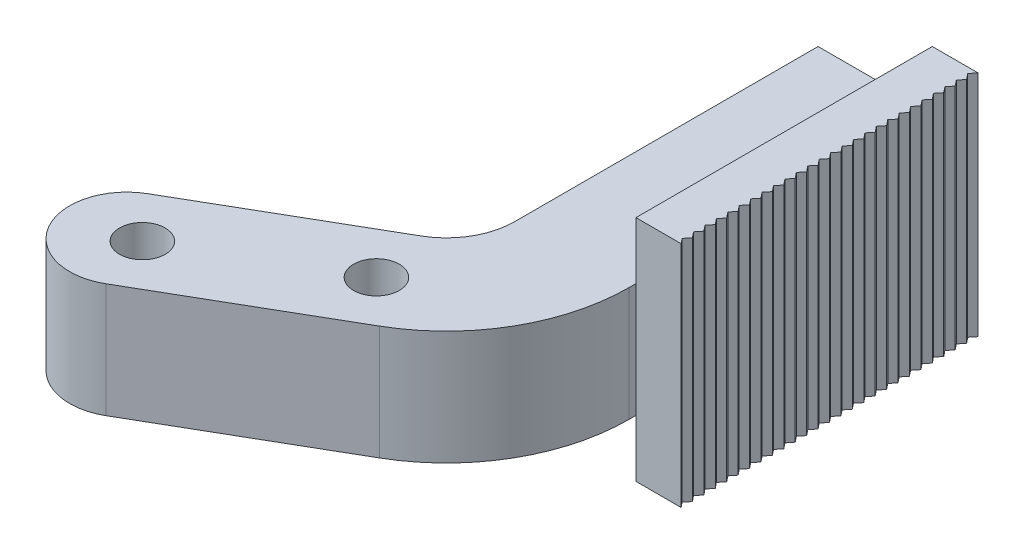
from build123d import *

# Parameters (mm, degrees)
SKETCH1_R           = 10
BOSS_EXTRUDE1_DEPTH = 50
FILLET1_RADIUS      = 25
FILLET1_LENGTH      = 50
SKETCH2_W           = 129.723894377
SKETCH2_H           = 100
BOSS_EXTRUDE2_DEPTH = 20
CUT_EXTRUDE1_DEPTH  = 240.757846963


with BuildPart() as part:
    # Sketch1 → Boss-Extrude1 (new body)
    with BuildSketch(Plane(origin=(0, 0, 0), x_dir=(1, 0, 0), z_dir=(0, 1, 0))):
        with BuildLine():
            Line((-39.067263876, -86.222925476), (-136.650566368, -142.562671438))
            Line((-136.650566368, -142.562671438), (-111.650566368, -185.863941628))
            Line((-111.650566368, -185.863941628), (-14.067263876, -129.524195665))
            ThreePointArc((-14.067263876, -129.524195665), (15.214768427, -100.242163363), (25.932736124, -60.242163363))
            Line((25.932736124, -60.242163363), (25.932736124, 72.437328562))
            Line((25.932736124, 72.437328562), (-24.067263876, 72.437328562))
            Line((-24.067263876, 72.437328562), (-24.067263876, -60.242163363))
            ThreePointArc((-24.067263876, -60.242163363), (-28.086501763, -75.242163363), (-39.067263876, -86.222925476))
        make_face()
        with Locations(Location((-98.169804255, -149.213306533, 0), (0, 0, 270))):
            Circle(SKETCH1_R, mode=Mode.SUBTRACT)
        with Locations(Location((-33.217898971, -111.713306533, 0), (0, 0, 270))):
            Circle(SKETCH1_R, mode=Mode.SUBTRACT)
    extrude(amount=BOSS_EXTRUDE1_DEPTH)

    # Fillet1: full round fillet: the end face becomes a half cylinder, R = half its width
    fillet1_face = Plane((-124.150566368, 25, 164.213306533), x_dir=(0, 1, 0), z_dir=(-0.866025403784, 0, 0.5))  # on the end face: x along it, z out of the body
    fillet1_slab = fillet1_face.offset(-FILLET1_RADIUS / 2) * Box(FILLET1_LENGTH, 2 * FILLET1_RADIUS, FILLET1_RADIUS, mode=Mode.PRIVATE)  # the body's end, R deep
    fillet1_round = Plane((-102.499931273, 25, 151.713306533), x_dir=(-0.866025403784, 0, 0.5), z_dir=(0, 1, 0)) * Cylinder(FILLET1_RADIUS, FILLET1_LENGTH, mode=Mode.PRIVATE)  # its axis R under the face
    add(fillet1_slab - fillet1_round, mode=Mode.SUBTRACT)

    # Sketch2 → Boss-Extrude2 (add)
    with BuildSketch(Plane(origin=(25.932736124, 0, 0), x_dir=(0, 0, -1), z_dir=(1, 0, 0))):
        with Locations((7.575381374, 25)):
            Rectangle(SKETCH2_W, SKETCH2_H)
    extrude(amount=BOSS_EXTRUDE2_DEPTH)

    # Sketch3 → Cut-Extrude1 (cut, through all)
    with BuildSketch(Plane(origin=(0, 75, 0), x_dir=(1, 0, 0), z_dir=(0, 1, 0))):
        Polygon((45.932736124, 67.437328562), (45.932736124, 72.437328562), (43.932736124, 69.937328562), align=None)
        Polygon((45.932736124, 62.437328562), (45.932736124, 67.437328562), (43.932736124, 64.937328562), align=None)
        Polygon((45.932736124, 57.437328562), (45.932736124, 62.437328562), (43.932736124, 59.937328562), align=None)
        Polygon((45.932736124, 52.437328562), (45.932736124, 57.437328562), (43.932736124, 54.937328562), align=None)
        Polygon((45.932736124, 47.437328562), (45.932736124, 52.437328562), (43.932736124, 49.937328562), align=None)
        Polygon((45.932736124, 42.437328562), (45.932736124, 47.437328562), (43.932736124, 44.937328562), align=None)
        Polygon((45.932736124, 37.437328562), (45.932736124, 42.437328562), (43.932736124, 39.937328562), align=None)
        Polygon((45.932736124, 32.437328562), (45.932736124, 37.437328562), (43.932736124, 34.937328562), align=None)
        Polygon((45.932736124, 27.437328562), (45.932736124, 32.437328562), (43.932736124, 29.937328562), align=None)
        Polygon((45.932736124, 22.437328562), (45.932736124, 27.437328562), (43.932736124, 24.937328562), align=None)
        Polygon((45.932736124, 17.437328562), (45.932736124, 22.437328562), (43.932736124, 19.937328562), align=None)
        Polygon((45.932736124, 12.437328562), (45.932736124, 17.437328562), (43.932736124, 14.937328562), align=None)
        Polygon((45.932736124, 7.437328562), (45.932736124, 12.437328562), (43.932736124, 9.937328562), align=None)
        Polygon((45.932736124, 2.437328562), (45.932736124, 7.437328562), (43.932736124, 4.937328562), align=None)
        Polygon((45.932736124, -2.562671438), (45.932736124, 2.437328562), (43.932736124, -0.062671438), align=None)
        Polygon((45.932736124, -7.562671438), (45.932736124, -2.562671438), (43.932736124, -5.062671438), align=None)
        Polygon((45.932736124, -12.562671438), (45.932736124, -7.562671438), (43.932736124, -10.062671438), align=None)
        Polygon((45.932736124, -22.562671438), (45.932736124, -17.562671438), (43.932736124, -20.062671438), align=None)
        Polygon((45.932736124, -27.562671438), (45.932736124, -22.562671438), (43.932736124, -25.062671438), align=None)
        Polygon((45.932736124, -32.562671438), (45.932736124, -27.562671438), (43.932736124, -30.062671438), align=None)
        Polygon((45.932736124, -37.562671438), (45.932736124, -32.562671438), (43.932736124, -35.062671438), align=None)
        Polygon((45.932736124, -42.562671438), (45.932736124, -37.562671438), (43.932736124, -40.062671438), align=None)
        Polygon((45.932736124, -47.562671438), (45.932736124, -42.562671438), (43.932736124, -45.062671438), align=None)
        Polygon((45.932736124, -57.286565815), (45.932736124, -52.562671438), (43.932736124, -55.062671438), (45.711851625, -57.286565815), align=None)
        Polygon((45.932736124, -57.562671438), (45.932736124, -62.562671438), (43.932736124, -60.062671438), align=None)
        Polygon((45.932736124, -12.562671438), (45.932736124, -17.562671438), (43.932736124, -15.062671438), align=None)
        Polygon((45.932736124, -47.562671438), (45.932736124, -52.562671438), (43.932736124, -50.062671438), align=None)
    extrude(amount=-CUT_EXTRUDE1_DEPTH, mode=Mode.SUBTRACT)


solid = part.part
